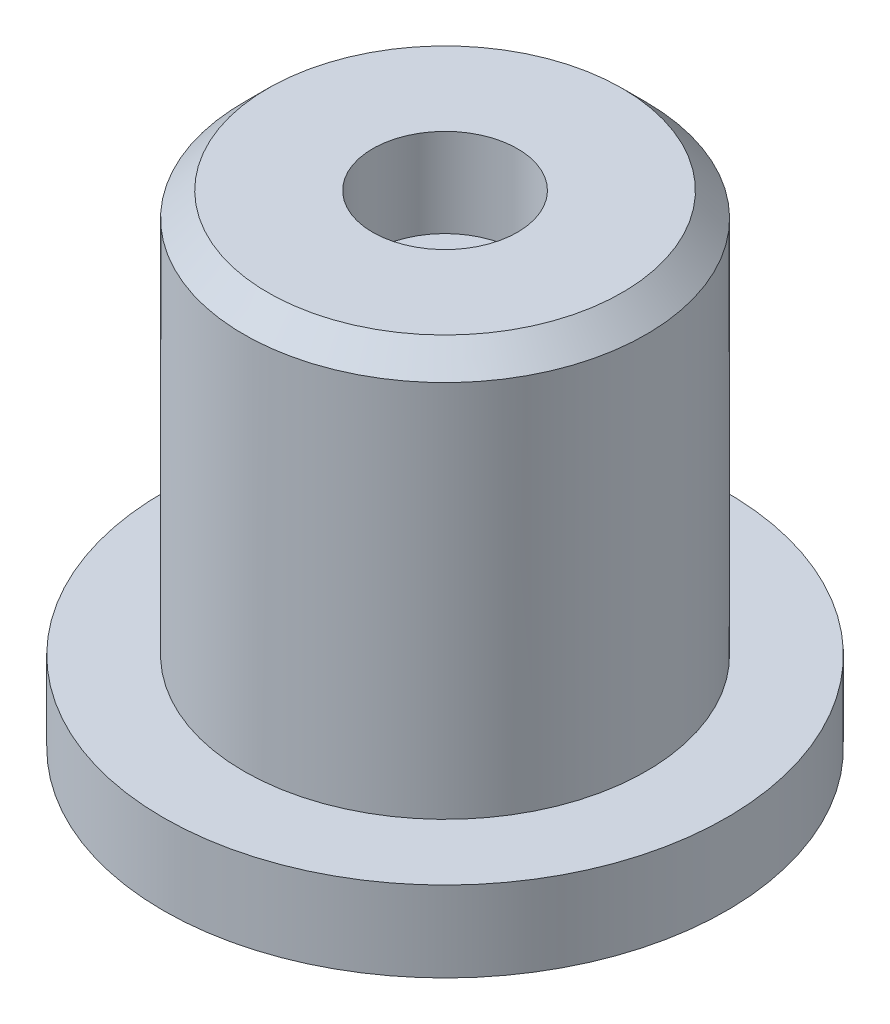
from build123d import *

# Parameters (mm, degrees)
SKETCH1_R           = 35
BOSS_EXTRUDE1_DEPTH = 10
SKETCH2_R           = 25
BOSS_EXTRUDE2_DEPTH = 50
CHAMFER1_SIZE       = 3
SKETCH3_R           = 9
CUT_EXTRUDE1_DEPTH  = 11
SKETCH4_R           = 5.5
CUT_EXTRUDE2_DEPTH  = 76


with BuildPart() as part:
    # Sketch1 → Boss-Extrude1 (new body)
    with BuildSketch(Plane(origin=(0, 0, 0), x_dir=(1, 0, 0), z_dir=(0, 1, 0))):
        with Locations(Location((0, 0, 0), (0, 0, 270))):
            Circle(SKETCH1_R)
    extrude(amount=BOSS_EXTRUDE1_DEPTH)

    # Sketch2 → Boss-Extrude2 (add)
    with BuildSketch(Plane(origin=(0, 10, 0), x_dir=(1, 0, 0), z_dir=(0, 1, 0))):
        with Locations(Location((0, 0, 0), (0, 0, 270))):
            Circle(SKETCH2_R)
    extrude(amount=BOSS_EXTRUDE2_DEPTH)

    # Chamfer1
    chamfer1_edges = [part.edges().sort_by_distance(p)[0] for p in [
        (0, 60, -25),
    ]]
    chamfer(chamfer1_edges, length=CHAMFER1_SIZE)

    # Sketch3 → Cut-Extrude1 (cut)
    with BuildSketch(Plane(origin=(0, 60, 0), x_dir=(1, 0, 0), z_dir=(0, 1, 0))):
        with Locations(Location((0, 0, 0), (0, 0, 270))):
            Circle(SKETCH3_R)
    extrude(amount=-CUT_EXTRUDE1_DEPTH, mode=Mode.SUBTRACT)

    # Sketch4 → Cut-Extrude2 (cut)
    with BuildSketch(Plane(origin=(0, 49, 0), x_dir=(1, 0, 0), z_dir=(0, 1, 0))):
        with Locations(Location((0, 0, 0), (0, 0, 270))):
            Circle(SKETCH4_R)
    extrude(amount=-CUT_EXTRUDE2_DEPTH, mode=Mode.SUBTRACT)


solid = part.part
